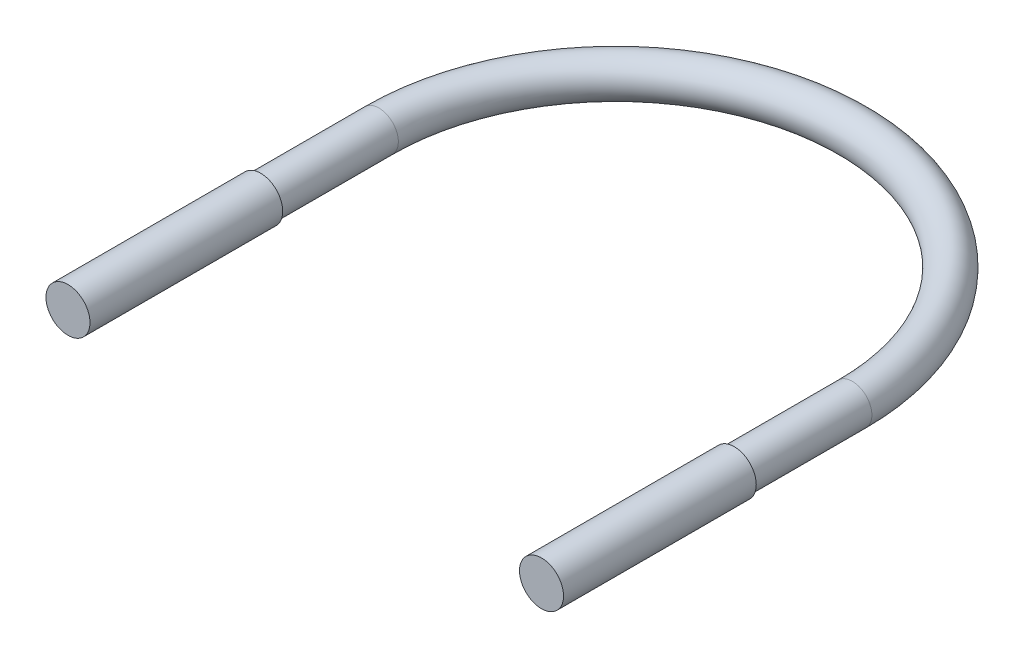
from build123d import *

# Parameters (mm, degrees)
SKETCH_1_R      = 3.55
SKETCH_3_R      = 4
EXTRUDE_1_DEPTH = 35


with BuildPart() as part:
    # 扫描1: sweep along a path in 草图2
    with BuildLine(Plane(origin=(0, 0, 0), x_dir=(1, 0, 0), z_dir=(0, 1, 0))) as sweep_1_path:
        Line((0, 0), (0, 56.45))
        ThreePointArc((0, 56.45), (43, 99.45), (86, 56.45))
        Line((86, 56.45), (86, 0))
    # 草图1 → 扫描1 (sweep)
    with BuildSketch(Plane.XY):
        Circle(SKETCH_1_R)
    sweep(path=sweep_1_path.line)

    # 草图3 → 凸台-拉伸1 (add)
    with BuildSketch(Plane.XY):
        Circle(SKETCH_3_R)
        with Locations((86, 0)):
            Circle(SKETCH_3_R)
    extrude(amount=-EXTRUDE_1_DEPTH)


solid = part.part
